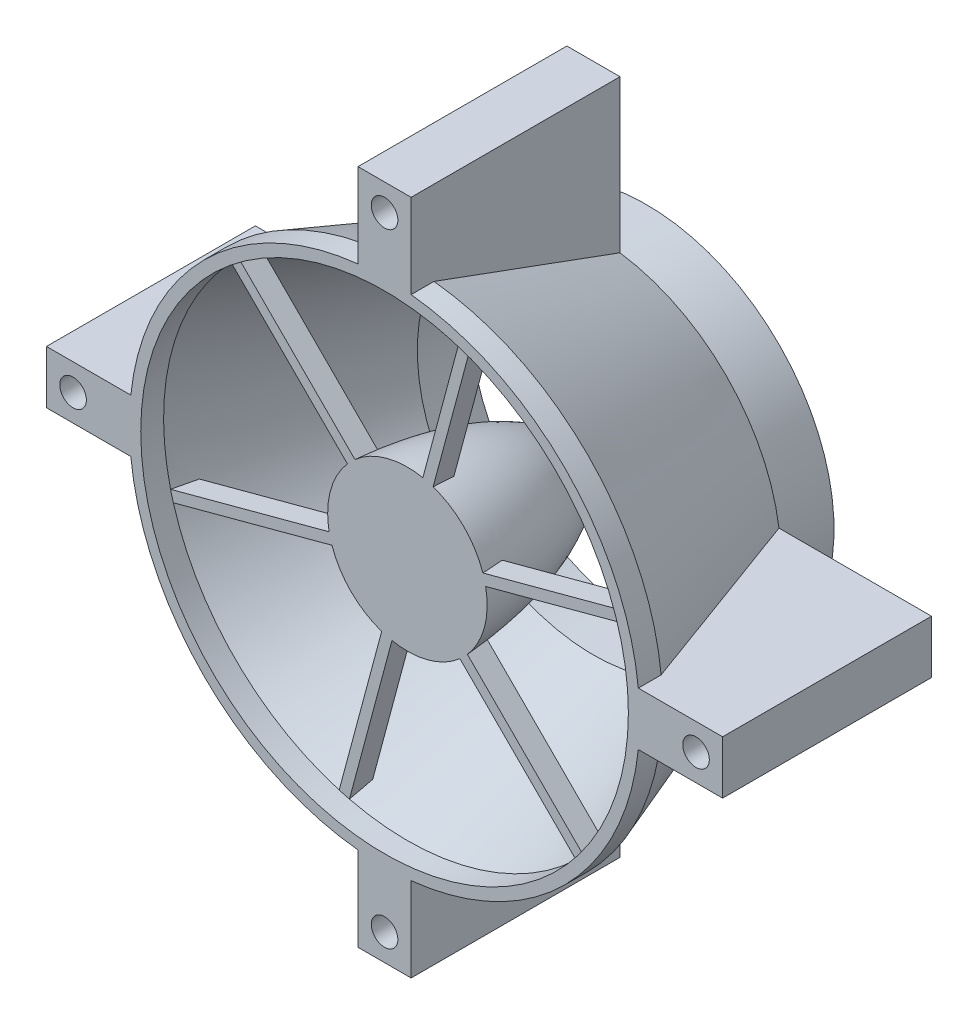
SolidWorks part; units mm, degrees
ref_plane "Front Plane" through (0, 0, 0) normal (0, 0, 1) x (1, 0, 0)
ref_plane "Top Plane" through (0, 0, 0) normal (0, 1, 0) x (1, 0, 0)
ref_plane "Right Plane" through (0, 0, 0) normal (1, 0, 0) x (0, 0, -1)
other "Configuration Table"
sketch "Sketch18" plane through (0, 0, 0) normal (0, 1, 0) x (1, 0, 0)
  line L0 (0, 0) -> (0, 105.5589) construction
  line L1 (0, 0) -> (-48, 0)
  line L2 (-48, 0) -> (-35.261, 35)
  line L3 (-35.261, 35) -> (0, 35)
  line L4 (0, 35) -> (0, 0)
  dimension "D1" = 48
  dimension "D2" = 70
  dimension "D3" = 35
revolve "Revolve1" add sketch "Sketch18" angle 360 about L0
shell "Shell2" thickness 2
ref_plane "Plane3" through (0, 63.6, 0) normal (0, 1, 0) x (1, 0, 0)
sketch "Sketch19" plane through (0, 0, 0) normal (0, 1, 0) x (1, 0, 0)
  line L0 (0, 0) -> (0, 49.4204) construction
sketch "Sketch20" plane through (0, 63.6, 0) normal (0, 1, 0) x (1, 0, 0)
  line L0 (0, 0) -> (0, 49.4204) construction
  line L1 (0, 0) -> (0, 49.4204) construction
  line L2 (-48, 0) -> (48, 0) construction
  line L3 (-5, 35) -> (5, 35)
  line L4 (-5, 35) -> (-5, 0)
  line L5 (-5, 0) -> (5, 0)
  line L6 (5, 35) -> (5, 0)
  line L7 (-5, 35) -> (5, 0) construction
  line L8 (-5, 0) -> (5, 35) construction
  line L9 (35.261, 35) -> (-35.261, 35) construction
  point P2 (0, 17.5)
  dimension "D1" = 10
extrude "Boss-Extrude10" add sketch "Sketch20" against normal up to surface (28.6953 mm away)
sketch "Sketch21" plane through (0, 0, -35) normal (0, 0, -1) x (-1, 0, 0)
  line L0 (0, 0) -> (0, 63.6) construction
  line L1 (27.1812, 63.6) -> (-27.1812, 63.6) construction
  line L3 (-5, 63.6) -> (5, 63.6) construction
  circle A0 centre (0, 58.6) radius 2.5
  dimension "D1" = 5
  dimension "D2" = 5
extrude "Cut-Extrude3" cut sketch "Sketch21" against normal through all
pattern_circular "CirPattern3" count 4 over 360 about axis through (0, 0, 0) along (0, 0, 1) of "Boss-Extrude10", "Cut-Extrude3"
sketch "Sketch22" plane through (0, 0, -35) normal (0, 0, -1) x (-1, 0, 0)
  circle A0 centre (0, 0) radius 35.261
  circle A1 centre (0, 0) radius 33.1327 construction
  circle A2 centre (0, 0) radius 33.1327
  dimension "D1" = 70.5221
extrude "Boss-Extrude11" add sketch "Sketch22" along normal blind 10
sketch "Sketch23" plane through (0, 0, 0) normal (0, 1, 0) x (1, 0, 0)
  line L0 (0, 0) -> (-15, 0)
  line L1 (-47.7389, 0) -> (-5, 0) construction
  line L2 (0, 0) -> (0, 35) construction
  line L3 (0, 0) -> (0, 49.4204) construction
  line L4 (0, 35) -> (0, 0)
  spline S0 degree 3 poles (-15, 0) (-14.1344, 12.4251) (-11.0616, 27.3666) (0, 35) knots 0 0 0 0 1 1 1 1
  dimension "D1" = 15
  dimension "D2" = 35
  dimension "D3" = 12.3176
  dimension "D4" = 5.9847
  dimension "D5" = 16.2434
  dimension "D6" = 29.2902
revolve "Revolve2" add sketch "Sketch23" angle 360 about L2
ref_plane "Plane4" through (0, 0, 0) normal (-0.7071, 0.7071, 0) x (0, 0, -1)
ref_plane "Plane5" through (-14.1421, 14.1421, 0) normal (-0.7071, 0.7071, 0) x (0, 0, -1)
sketch "Sketch24" plane through (-14.1421, 14.1421, 0) normal (-0.7071, 0.7071, 0) x (0, 0, -1)
  line L0 (0, 0) -> (49.4204, 0) construction
  line L1 (0, 0) -> (49.4204, 0) construction
  line L2 (0, 15) -> (0, -15) construction
  line L3 (0, 15) -> (0, -15) construction
  line L5 (4, 1) -> (0, 1)
  line L6 (4, 1) -> (4, -1)
  line L7 (4, -1) -> (0, -1)
  line L8 (0, 1) -> (0, -1)
  line L9 (4, 1) -> (0, -1) construction
  line L10 (4, -1) -> (0, 1) construction
  point P4 (2, 0)
  dimension "D1" = 2
  dimension "D2" = 4
extrude "Boss-Extrude12" add sketch "Sketch24" along normal up to next and the other way up to next
pattern_circular "CirPattern4" count 6 over 360 about axis through (0, 0, 0) along (0, 0, 1) of "Boss-Extrude12"
sketch "Sketch25" plane through (0, 0, 0) normal (0, 0, 1) x (1, 0, 0)
  line L12 (-47.7389, 5) -> (-63.6, 5)
  line L13 (-47.7389, 5) -> (-63.6, 5)
  line L14 (-63.6, 5) -> (-63.6, -5)
  line L15 (-63.6, 5) -> (-63.6, -5)
  line L16 (-63.6, -5) -> (-47.7389, -5)
  line L17 (-63.6, -5) -> (-47.7389, -5)
  line L18 (-5, -47.7389) -> (-5, -63.6)
  line L19 (-5, -47.7389) -> (-5, -63.6)
  line L20 (-5, -63.6) -> (5, -63.6)
  line L21 (5, 47.7389) -> (5, 63.6)
  line L22 (5, 63.6) -> (-5, 63.6)
  line L23 (-5, 63.6) -> (-5, 47.7389)
  line L33 (5, 47.7389) -> (5, 63.6)
  line L34 (5, 63.6) -> (-5, 63.6)
  line L35 (-5, 63.6) -> (-5, 47.7389)
  line L36 (-5, -63.6) -> (5, -63.6)
  line L37 (5, -63.6) -> (5, -47.7389)
  line L38 (5, -63.6) -> (5, -47.7389)
  line L39 (47.7389, -5) -> (63.6, -5)
  line L40 (47.7389, -5) -> (63.6, -5)
  line L41 (63.6, -5) -> (63.6, 5)
  line L42 (63.6, -5) -> (63.6, 5)
  line L43 (63.6, 5) -> (47.7389, 5)
  line L44 (63.6, 5) -> (47.7389, 5)
  circle A0 centre (0, 0) radius 45.8716
  arc A1 (-33.1355, 31.7213) -> (-44.5569, -10.9037) centre (0, 0) ccw construction
  arc A4 (-5, 47.7389) -> (-47.7389, 5) centre (0, 0) ccw
  arc A7 (-47.7389, -5) -> (-5, -47.7389) centre (0, 0) ccw
  arc A8 (-5, 47.7389) -> (-47.7389, 5) centre (0, 0) ccw
  arc A12 (-47.7389, -5) -> (-5, -47.7389) centre (0, 0) ccw
  arc A13 (5, -47.7389) -> (47.7389, -5) centre (0, 0) ccw
  arc A14 (5, -47.7389) -> (47.7389, -5) centre (0, 0) ccw
  arc A15 (47.7389, 5) -> (5, 47.7389) centre (0, 0) ccw
  arc A16 (47.7389, 5) -> (5, 47.7389) centre (0, 0) ccw
  dimension "D1" = 0
extrude "Boss-Extrude13" add sketch "Sketch25" along normal blind 4.3
sketch "Sketch26" plane through (0, 0, 4.3) normal (0, 0, 1) x (1, 0, 0)
  circle A0 centre (-58.6, 0) radius 2.5 construction
  circle A1 centre (-58.6, 0) radius 2.5
extrude "Cut-Extrude4" cut sketch "Sketch26" against normal through all
sketch "Sketch27" plane through (0, 0, 4.3) normal (0, 0, 1) x (1, 0, 0)
  circle A0 centre (0, 58.6) radius 2.5 construction
  circle A1 centre (0, 58.6) radius 2.5
extrude "Cut-Extrude5" cut sketch "Sketch27" against normal through all
sketch "Sketch28" plane through (0, 0, 4.3) normal (0, 0, 1) x (1, 0, 0)
  circle A0 centre (0, -58.6) radius 2.5 construction
  circle A1 centre (58.6, 0) radius 2.5 construction
  circle A2 centre (0, -58.6) radius 2.5
  circle A3 centre (58.6, 0) radius 2.5
extrude "Cut-Extrude6" cut sketch "Sketch28" against normal through all
